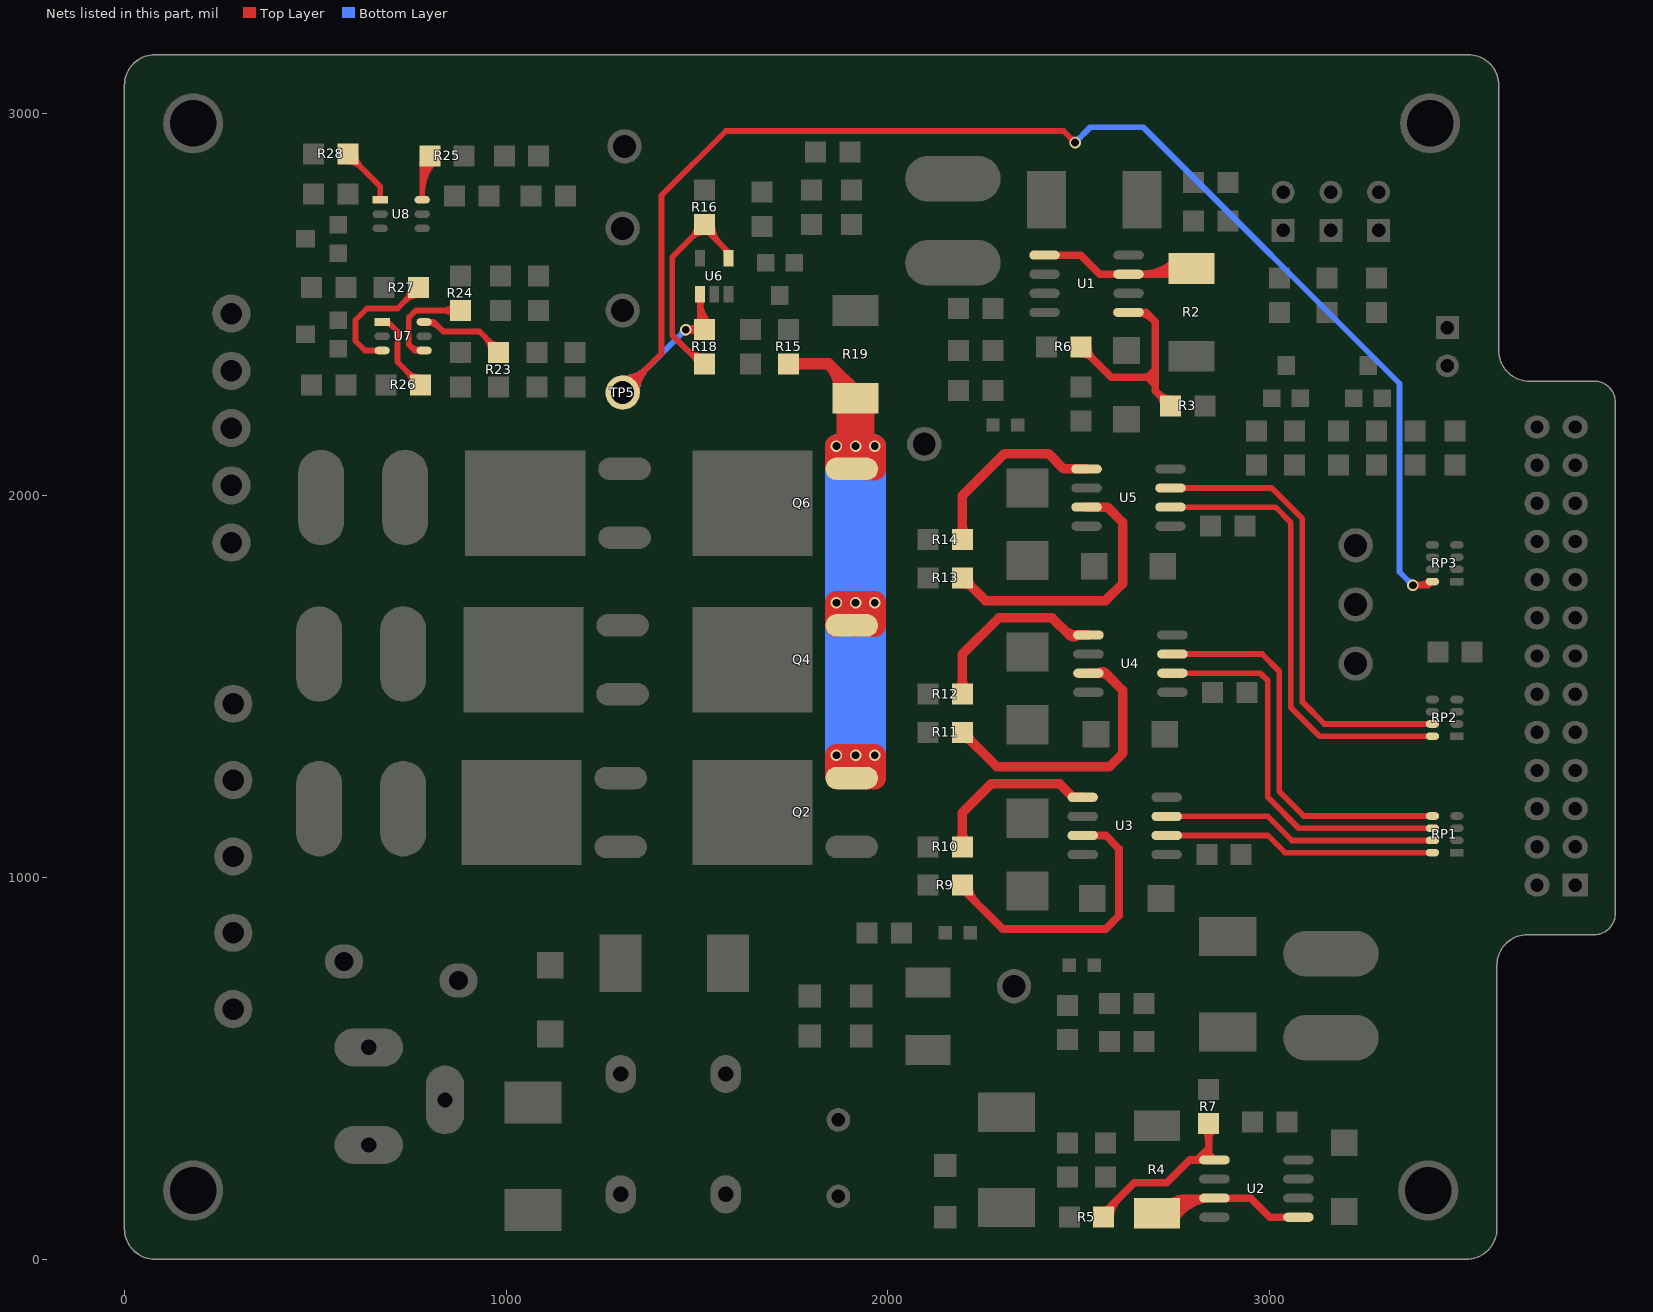
[diagram p0: the nets of this part, all layers, seen from the top]
# Altium PCB MISC103926.PcbDoc (part 4 of 4)
Units mil, origin at the board's own origin, x right, y up, seen from the top; angles counter-clockwise.
Board outline 3905 x 3155 mil, 4 copper layers (Top Layer, GND1, GND2, Bottom Layer); 132 components, 84 nets, 362 pads, 268 vias.

## Via types
v1: diameter 30, hole 20, Top Layer to Bottom Layer, 268 vias

## Nets (pads, with @x,y where several pads share a name; then routed paths per layer and width w, separated by ;. In a path a pad name is that pad's centre, name@x,y a point inside that pad or via, vN(x,y) a via of type N, cw(c..) or ccw(c..) an arc to the next point about the centre after c; other vN are vias at no path point) (continued)
NetQ2_3: Q2.3 Q4.3 Q6.3 R15.2 R19.2 | length 4611.5
  Top Layer w30: R15.2@1740,2345 1845,2345 ; R15.2@1748.84,2336.16 cw(c1770.18,2314.82) 1770.18,2345 cw(c1770.18,2375.18) R15.2@1748.84,2353.84 ; R19.2@1870.51,2260.02 ccw(c1778.82,2278.82) 1845,2345 ; 1884.41,2305.59 cw(c1844.23,2265.41) R19.2@1899.9,2254 ; R19.2@1935,2255 1845,2345
  Top Layer w60: Q2.3@1865,1265 v1(1865,1320) ; Q4.3@1865,1660 v1(1865,1720) ; Q6.3@1865,2075 v1(1865,2130) ; Q2.3@1915,1265 v1(1915,1320) v1(1865,1320) ; Q4.3@1915,1660 v1(1915,1720) v1(1865,1720) ; Q6.3@1915,2075 v1(1915,2130) v1(1865,2130) ; Q2.3@1944.7,1259.98 ccw(c1895.71,1308.98) v1@1965,1308.98 ; Q4.3@1944.7,1659.98 ccw(c1895.71,1708.98) v1@1965,1708.98 ; Q6.3@1944.7,2069.98 ccw(c1895.71,2118.98) v1@1965,2118.98 ; Q2.3@1965,1260 v1(1965,1320) v1(1865,1320) ; Q4.3@1965,1660 v1(1965,1720) v1(1865,1720) ; Q6.3@1965,2070 v1(1965,2130) v1(1865,2130)
  Top Layer w100: v1(1915,2130) R19.2@1915,2245
  Bottom Layer w60: v1@1865,1330 v1(1865,1320) ; 1865,1370 1865,1410 ; 1865,1600 1865,1620 ; 1865,1635 1865,1670 ; v1(1865,1720) v1(1965,1720) v1@1950,1720 ; 1865,1770 1865,1805 ; v1(1915,1320) v1(1915,2130) v1(1865,2130) ; v1(1865,1320) v1(1865,2130) ; v1(1865,1320) v1(1965,1320) v1(1965,2130) v1(1865,2130)
NetR2_2: R2.2 U1.1 U1.7 | length 568.2
  Top Layer w20: U1.1@2410,2630 2505,2630 2555,2580 U1.7@2630,2580 2780,2580 R2.2@2795,2595 ; U1.7@2666.36,2580 ccw(c2666.36,2703.64) R2.2@2753.79,2616.21 ; 2714.64,2580 ccw(c2714.64,2655.36) R2.2@2767.93,2602.07
NetR3_1: R3.1 R6.1 U1.5 | length 810.4
  Top Layer w20: R6.1@2505,2372.5 cw(c2505,2330.25) 2534.87,2360.13 cw(c2564.75,2390) R6.1@2522.5,2390 ; R6.1@2505,2390 2585,2310 2675,2310 ; U1.5@2600,2480 U1.5@2630,2480 2675,2480 2700,2455 2700,2310 ; U1.5@2658,2478 cw(c2658,2432.13) 2690.44,2464.56 ; 2700,2290 2680,2310 ; 2700,2330 2680,2310 ; R3.1@2722.5,2235 ccw(c2680.25,2235) 2710.13,2264.87 ccw(c2740,2294.75) R3.1@2740,2252.5 ; R3.1@2740,2235 2700,2275 2700,2310 ; 2675,2310 2700,2310 ; 2675,2310 2680,2310 ; 2675,2310 2680,2310
NetR4_2: R4.2 U2.1 U2.7 | length 790.7
  Top Layer w20: R4.2@2705,120 2735,120 2775,160 ; R4.2@2716.65,125.5 cw(c2780.71,83.27) 2780.71,160 ; R4.2@2732.99,148.92 ccw(c2744.48,190.51) 2775,160 ; R4.2@2733.35,114.5 cw(c2817.85,58.78) U2.7@2817.85,160 ; R4.2@2750.05,103.49 cw(c2854.99,34.3) U2.7@2855,160 ; R4.2@2755,120 cw(c2803.29,120) 2769.14,154.14 ; U2.1@3075,110 3000,110 2950,160 U2.7@2855,160 ; 2775,160 U2.7@2855,160
NetR5_1: R5.1 R7.1 U2.5 | length 706.3
  Top Layer w20: R5.1@2565,110 2565,120 2645,200 2730,200 2790,260 U2.5@2855,260 2840,275 ; R5.1@2582.5,110 cw(c2648.89,110) 2601.95,156.95 ; 2810,260 2840,290 ; U2.5@2825.8,261.6 ccw(c2804.5,290) 2840,290 ; U2.5@2827,262 ccw(c2827,275) 2840,275 ; R7.1@2827.63,342.63 cw(c2797.75,312.75) 2840,312.75 cw(c2882.25,312.75) R7.1@2852.37,342.63 ; U2.5@2828.99,260.16 cw(c2866.85,263.15) 2840,290 ; R7.1@2840,355 2840,290 ; 2840,275 2840,290
NetR9_1: R9.1 U3.7 | length 814.6
  Top Layer w20: R9.1@2195,980 2195,970 2300,865 2570,865 2605,900 2605,1075 2570,1110 U3.7@2510,1110 ; R9.1@2212.5,980 ccw(c2278.89,980) 2231.95,933.05
NetR10_1: R10.1 U3.5 | length 507.4
  Top Layer w25: R10.1@2184.39,1090.61 ccw(c2158.79,1116.21) 2195,1116.21 ccw(c2231.21,1116.21) R10.1@2205.61,1090.61 ; R10.1@2195,1080 2195,1170 2270,1245 2450,1245 2485,1210 U3.5@2510,1210
NetR11_1: R11.1 U4.7 | length 852.7
  Top Layer w25: R11.1@2195,1365 cw(c2195,1328.79) 2220.61,1354.39 cw(c2246.21,1380) R11.1@2210,1380 ; R11.1@2195,1380 2285,1290 2580,1290 2615,1325 2615,1490 2570,1535 ; U4.7@2525,1535 2570,1535 ; U4.7@2552.66,1535.37 cw(c2561.14,1526.14) 2570,1535 ; U4.7@2553,1535.5 cw(c2553,1495.67) 2581.17,1523.83
NetR12_1: R12.1 U4.5 | length 615.4
  Top Layer w25: R12.1@2184.39,1490.61 ccw(c2158.79,1516.21) 2195,1516.21 ccw(c2231.21,1516.21) R12.1@2205.61,1490.61 ; R12.1@2195,1480 2195,1585 2290,1680 2430,1680 2475,1635 ; 2460.3,1649.7 ccw(c2497,1686.41) U4.5@2497,1634.5 ; U4.5@2497.34,1634.64 cw(c2486.36,1646.36) 2475,1635 ; U4.5@2525,1635 2475,1635
NetR13_1: R13.1 U5.7 | length 791.9
  Top Layer w25: R13.1@2195,1770 cw(c2195,1733.79) 2220.61,1759.39 cw(c2246.21,1785) R13.1@2210,1785 ; R13.1@2195,1785 2255,1725 2570,1725 2615,1770 2615,1930 2575,1970 U5.7@2520,1970
NetR14_1: R14.1 U5.5 | length 559
  Top Layer w25: R14.1@2184.39,1895.61 ccw(c2158.79,1921.21) 2195,1921.21 ccw(c2231.21,1921.21) R14.1@2205.61,1895.61 ; R14.1@2195,1885 2195,2000 2305,2110 2420,2110 2460,2070 U5.5@2520,2070
NetR16_1: R16.1 R18.2 U6.4 | length 851.7
  Top Layer w15: 1468.79,2386.21 ccw(c1520,2437.43) R18.2@1520,2365 ; R18.2@1492.93,2362.07 cw(c1475.86,2345) R18.2@1500,2345 ; R18.2@1494.39,2360.61 ccw(c1520,2386.21) R18.2@1520,2350 ; R16.1@1500,2710 cw(c1451.72,2710) 1485.86,2675.86 cw(c1520,2641.72) 1520,2690 cw(c1520,2665.86) R16.1@1537.07,2682.93 ; R18.2@1520,2345 1510,2345 1435,2420 1435,2625 1515,2705 1582.4,2637.6 U6.4@1582.4,2622.24 ; R16.1@1525,2710 ccw(c1561.21,2710) R16.1@1535.61,2684.39 ; R16.1@1540,2710 ccw(c1612.43,2710) 1561.21,2658.79 ; 1568.77,2651.23 cw(c1548.64,2631.1) U6.4@1577.11,2631.1
NetR18_1: R18.1 RP3.8 TP5.1 U6.1 | length 4789.7
  Top Layer w15: TP5.1@1305,2270 1407,2372 1407,2786.64 1575.36,2955 2460,2955 v1(2490,2925) ; TP5.1@1305,2292.5 ccw(c1305,2346.82) 1343.41,2308.41 ccw(c1381.82,2270) TP5.1@1327.5,2270 ; TP5.1@1305,2307.5 ccw(c1305,2398.03) 1369.02,2334.02 ccw(c1433.03,2270) TP5.1@1342.5,2270 ; v1(1470,2435) R18.1@1520,2435 1507.6,2447.4 U6.1@1507.6,2527.76 ; v1@1473.75,2428.5 cw(c1483.56,2411.51) 1488.64,2430.47 ; v1@1473.75,2441.5 ccw(c1483.56,2458.49) 1488.64,2439.53 ; v1@1475.3,2429.7 cw(c1488.11,2416.89) 1488.11,2435 cw(c1488.11,2453.11) v1@1475.3,2440.3 ; v1@1476.5,2431.25 cw(c1490.86,2422.95) 1486.57,2438.98 ; v1@1476.5,2438.75 ccw(c1490.86,2447.05) 1486.57,2431.02 ; R18.1@1505.86,2420.86 ccw(c1471.72,2386.72) 1471.72,2435 ccw(c1471.72,2483.28) R18.1@1505.86,2449.14 ; 1507.6,2477.01 ccw(c1562.01,2477.01) R18.1@1523.54,2438.54 ; U6.1@1507.6,2513.22 ccw(c1598.22,2513.22) R18.1@1534.14,2449.14 ; 1510.41,2502.75 cw(c1527.6,2507.35) U6.1@1512.18,2516.25 ; v1@2482.5,2925 ccw(c2464.39,2925) 2477.2,2937.8 ccw(c2490,2950.61) v1@2490,2932.5 ; v1(3375,1765) 3416,1765 RP3.8@3426,1775 ; v1@3378.75,1771.5 ccw(c3393.69,1797.37) 3401.42,1768.51 ; v1@3380.3,1759.7 cw(c3393.11,1746.89) 3393.11,1765 cw(c3393.11,1783.11) v1@3380.3,1770.3 ; v1@3388.32,1765 ccw(c3388.32,1805.18) RP3.8@3416.73,1776.77
  Bottom Layer w15: TP5.1@1305,2270 v1(1470,2435) ; TP5.1@1305,2292.5 ccw(c1305,2346.82) 1343.41,2308.41 ccw(c1381.82,2270) TP5.1@1327.5,2270 ; TP5.1@1305,2307.5 ccw(c1305,2398.03) 1369.02,2334.02 ccw(c1433.03,2270) TP5.1@1342.5,2270 ; v1@1462.5,2435 cw(c1444.39,2435) 1457.2,2422.2 cw(c1470,2409.39) v1@1470,2427.5 ; v1(2490,2925) 2530,2965 2668.79,2965 3340,2293.79 3340,1800 v1(3375,1765) ; v1@2490,2932.5 ccw(c2490,2950.61) 2502.8,2937.8 ccw(c2515.61,2925) v1@2497.5,2925 ; v1@3367.5,1765 ccw(c3349.39,1765) 3362.2,1777.8 ccw(c3375,1790.61) v1@3375,1772.5
NetR23_2: R23.2 U7.6 | length 342.2
  Top Layer w15: U7.6@785,2455 810,2455 835,2430 930,2430 R23.2@985,2375 ; U7.6@795,2452.5 cw(c795,2410.25) 824.88,2440.12 ; 942.32,2417.68 cw(c899.64,2375) R23.2@960,2375 ; 954.39,2405.61 ccw(c980,2431.21) R23.2@980,2395
NetR24_2: R24.2 U7.4 | length 369.5
  Top Layer w15: U7.4@774.98,2382.7 cw(c774.7,2424.7) 745,2395 ; U7.4@785,2380.2 759.8,2380.2 745,2395 ; R24.2@865.86,2470.86 ccw(c831.72,2436.72) 831.72,2485 ccw(c831.72,2533.28) R24.2@865.86,2499.14 ; R24.2@880,2485 763.28,2485 745,2466.72 745,2395
NetR25_2: R25.2 U8.6 | length 312.6
  Top Layer w15: U8.6@780,2775 780,2870 R25.2@800,2890 ; 780,2793.43 cw(c896.57,2793.43) R25.2@814.14,2875.86 ; 780,2829.64 cw(c860.36,2829.64) R25.2@803.54,2886.46 ; R25.2@780,2865.86 cw(c824.14,2865.86) R25.2@792.93,2897.07
NetR26_1: R26.1 U7.1 | length 305.3
  Top Layer w15: U7.1@675,2455 690,2455 715,2430 715,2350 R26.1@775,2290 ; U7.1@685,2452.5 cw(c685,2434.39) 697.8,2447.2 ; R26.1@755,2290 ccw(c706.72,2290) 740.86,2324.14 ccw(c775,2358.28) R26.1@775,2310
NetR27_1: R27.1 U7.3 | length 411.3
  Top Layer w15: U7.3@675,2380.2 629.8,2380.2 605,2405 605,2460 635,2490 715,2490 R27.1@770,2545 ; R27.1@750,2545 cw(c701.72,2545) 735.86,2510.86 cw(c770,2476.72) R27.1@770,2525
NetR28_1: R28.1 U8.1 | length 231.1
  Top Layer w15: R28.1@585,2875 cw(c585,2826.72) 619.14,2860.86 cw(c653.28,2895) R28.1@605,2895 ; R28.1@585,2895 670,2810 U8.1@670,2775
NetRP1_5: RP1.5 U4.3 | length 1041.1
  Top Layer w15: U4.3@2745,1585 2980,1585 3025,1540 3025,1225 3089,1161 RP1.5@3426,1161
NetRP1_6: RP1.6 U4.2 | length 1027.8
  Top Layer w15: U4.2@2745,1535 2975,1535 2995,1515 2995,1210 3076,1129 RP1.6@3426,1129
NetRP1_7: RP1.7 U3.3 | length 722.1
  Top Layer w15: U3.3@2730,1160 2995,1160 3058,1097 RP1.7@3426,1097
NetRP1_8: RP1.8 U3.2 | length 714.6
  Top Layer w15: U3.2@2730,1110 2995,1110 3040,1065 RP1.8@3426,1065
NetRP2_7: RP2.7 U5.3 | length 1223.2
  Top Layer w15: U5.3@2740,2020 3005,2020 3085,1940 3085,1460 3143,1402 RP2.7@3426,1402
NetRP2_8: RP2.8 U5.2 | length 1218.6
  Top Layer w15: U5.2@2740,1970 3015,1970 3055,1930 3055,1445 3130,1370 RP2.8@3426,1370
pads on no net: JP1.7 JP1.8 JP1.9 JP1.14 JP1.15 JP1.17 JP1.18 JP1.19 U1.8 U2.8 U8.4

## Polygon pours and split planes (outlines as drawn)
GND on Bottom Layer "Top Layer-No Net" (solid, remove dead copper, pour order 2): 1456.72,-4.27 1456.72,655.73 1206.72,655.73 1206.72,950.73 2506.72,950.73 2506.72,2200.73 926.72,2200.73 806.72,2200.73 356.72,1750.73 346.72,1740.73 1.72,1740.73 1.72,3145.73 -8.28,3155.73 -3.28,3160.73 3911.72,3160.73 3911.72,5.73 3916.72,0.73
GND on Top Layer "Top Layer-No Net 1" (solid, remove dead copper, pour order 6): 1453.51,-8.28 1453.51,641.72 1203.51,641.72 1203.51,946.72 2158.51,946.72 2158.51,2201.72 453.51,2201.72 448.51,2201.72 383.51,2136.72 378.51,2131.72 378.51,1936.72 373.51,1936.72 173.51,1736.72 -46.49,1736.72 -46.49,3186.72 -41.49,3191.72 3958.51,3191.72 3958.51,-13.28
GND on GND2 (split plane): 80,3134.9 3520,3134.9 3520.59,3134.96 3526.72,3134.62 3533.35,3133.49 3539.81,3131.63 3546.03,3129.05 3551.92,3125.8 3557.41,3121.91 3562.42,3117.42 3566.91,3112.41 3570.8,3106.92 3574.05,3101.03 3576.63,3094.81 3578.49,3088.35 3579.62,3081.72 3579.96,3075.59 3579.9,3075 3579.9,2380 3579.91,2379.97 3580.29,2371.28 3581.43,2362.62 3583.32,2354.09 3585.94,2345.77 3589.28,2337.7 3593.31,2329.95 3598.01,2322.59 3603.32,2315.66 3609.22,2309.22 3615.66,2303.32 3622.59,2298.01 3629.95,2293.31 3637.7,2289.28 3645.77,2285.94 3654.09,2283.32 3662.62,2281.43 3671.28,2280.29 3679.97,2279.91 3680,2279.9 3850,2279.9 3850.44,2279.95 3854.57,2279.68 3859.05,2278.78 3863.38,2277.31 3867.49,2275.29 3871.29,2272.75 3874.73,2269.73 3877.75,2266.29 3880.29,2262.49 3882.31,2258.38 3883.78,2254.05 3884.68,2249.57 3884.95,2245.44 3884.9,2245 3884.9,905 3884.95,904.56 3884.68,900.43 3883.78,895.95 3882.31,891.62 3880.29,887.51 3877.75,883.71 3874.73,880.27 3871.29,877.25 3867.49,874.71 3863.38,872.69 3859.05,871.22 3854.57,870.32 3850.44,870.05 3850,870.1 3675,870.1 3674.97,870.09 3666.28,869.71 3657.62,868.57 3649.09,866.68 3640.77,864.06 3632.7,860.72 3624.95,856.69 3617.59,851.99 3610.66,846.68 3604.22,840.78 3598.32,834.34 3593.01,827.41 3588.31,820.05 3584.28,812.3 3580.94,804.23 3578.32,795.91 3576.43,787.38 3575.29,778.72 3574.91,770.03 3574.9,770 3574.9,80 3574.96,79.41 3574.62,73.28 3573.49,66.65 3571.63,60.18 3569.05,53.97 3565.8,48.08 3561.91,42.59 3557.42,37.58 3552.41,33.09 3546.92,29.2 3541.03,25.95 3534.81,23.37 3528.35,21.51 3521.72,20.38 3515.59,20.04 3515,20.1 80,20.1 79.41,20.04 73.28,20.38 66.65,21.51 60.18,23.37 53.97,25.95 48.08,29.2 42.59,33.09 37.58,37.58 33.09,42.59 29.2,48.08 25.95,53.97 23.37,60.19 21.51,66.65 20.38,73.28 20.04,79.41 20.1,80 20.1,3075 20.04,3075.59 20.38,3081.72 21.51,3088.35 23.37,3094.81 25.95,3101.03 29.2,3106.92 33.09,3112.41 37.58,3117.42 42.59,3121.91 48.08,3125.8 53.97,3129.05 60.19,3131.63 66.65,3133.49 73.28,3134.62 79.41,3134.96
GND on GND1 (split plane): 80,3134.9 3520,3134.9 3520.59,3134.96 3526.72,3134.62 3533.35,3133.49 3539.81,3131.63 3546.03,3129.05 3551.92,3125.8 3557.41,3121.91 3562.42,3117.42 3566.91,3112.41 3570.8,3106.92 3574.05,3101.03 3576.63,3094.81 3578.49,3088.35 3579.62,3081.72 3579.96,3075.59 3579.9,3075 3579.9,2380 3579.91,2379.97 3580.29,2371.28 3581.43,2362.62 3583.32,2354.09 3585.94,2345.77 3589.28,2337.7 3593.31,2329.95 3598.01,2322.59 3603.32,2315.66 3609.22,2309.22 3615.66,2303.32 3622.59,2298.01 3629.95,2293.31 3637.7,2289.28 3645.77,2285.94 3654.09,2283.32 3662.62,2281.43 3671.28,2280.29 3679.97,2279.91 3680,2279.9 3850,2279.9 3850.44,2279.95 3854.57,2279.68 3859.05,2278.78 3863.38,2277.31 3867.49,2275.29 3871.29,2272.75 3874.73,2269.73 3877.75,2266.29 3880.29,2262.49 3882.31,2258.38 3883.78,2254.05 3884.68,2249.57 3884.95,2245.44 3884.9,2245 3884.9,905 3884.95,904.56 3884.68,900.43 3883.78,895.95 3882.31,891.62 3880.29,887.51 3877.75,883.71 3874.73,880.27 3871.29,877.25 3867.49,874.71 3863.38,872.69 3859.05,871.22 3854.57,870.32 3850.44,870.05 3850,870.1 3675,870.1 3674.97,870.09 3666.28,869.71 3657.62,868.57 3649.09,866.68 3640.77,864.06 3632.7,860.72 3624.95,856.69 3617.59,851.99 3610.66,846.68 3604.22,840.78 3598.32,834.34 3593.01,827.41 3588.31,820.05 3584.28,812.3 3580.94,804.23 3578.32,795.91 3576.43,787.38 3575.29,778.72 3574.91,770.03 3574.9,770 3574.9,80 3574.96,79.41 3574.62,73.28 3573.49,66.65 3571.63,60.18 3569.05,53.97 3565.8,48.08 3561.91,42.59 3557.42,37.58 3552.41,33.09 3546.92,29.2 3541.03,25.95 3534.81,23.37 3528.35,21.51 3521.72,20.38 3515.59,20.04 3515,20.1 80,20.1 79.41,20.04 73.28,20.38 66.65,21.51 60.18,23.37 53.97,25.95 48.08,29.2 42.59,33.09 37.58,37.58 33.09,42.59 29.2,48.08 25.95,53.97 23.37,60.19 21.51,66.65 20.38,73.28 20.04,79.41 20.1,80 20.1,3075 20.04,3075.59 20.38,3081.72 21.51,3088.35 23.37,3094.81 25.95,3101.03 29.2,3106.92 33.09,3112.41 37.58,3117.42 42.59,3121.91 48.08,3125.8 53.97,3129.05 60.19,3131.63 66.65,3133.49 73.28,3134.62 79.41,3134.96

## Keep-outs
Keep-Out Layer:
  the board outline again, w10

## Other copper
Top Layer:
  rectangle net +24V: 900,1160 1190,1970
Bottom Layer:
  rectangle net MT_PV: 790,1450 1410,1755
  rectangle net MT_PU: 790,1045 1410,1350
  rectangle net MT_PW: 795,1865 1415,2150

## Silkscreen, mask and mechanical layers (free items; w line width, h text height)
Top Overlay:
  circle w16: c343,161 r5
  lines w10: 328.35,141.45 cw(c343.54,161.31) 359.03,141.69
  lines w12: 344,81 344,153 ; 344,188 344,259
  text "W" at 445,2425 h100 r90
  text "V" at 450,2320 h100 r90
  text "U" at 445,2180 h100 r90
  text "GND" at 450,1960 h100 r90
  text "5V" at 450,1805 h100 r90
  text "W" at 445,1400 h100 r90
  text "V" at 445,1225 h100 r90
  text "U" at 440,1035 h100 r90
  text "24V" at 440,825 h100 r90
  text "GND" at 440,505 h100 r90
  text "2013/4/5" at 3525,455 h80 r90
  text "BLDC Driver V1.00" at 3420,310 h80 r90
  text "-" at 327,246 h60 r90
  text "+24V" at 440,90 h80 r90
  text "+" at 300,73 h60
Bottom Overlay:
  lines w10: 3315,1035 3585,1035 ; 3315,1135 3585,1135 ; 3315,1240 3585,1240 ; 3315,1340 3585,1340 ; 3315,1440 3585,1440 ; 3315,1540 3585,1540 ; 3315,1640 3585,1640 ; 3315,1740 3585,1740 ; 3315,1835 3585,1835 ; 3315,1940 3585,1940 ; 3315,2035 3585,2035 ; 3315,2140 3585,2140 ; 3450,930 3450,2235 ; 3315,925 3315,2235 3585,2235 3585,925 3315,925
  text "GND" at 3435,2175 h40
  text "5V" at 3570,2175 h40
  text "A_MW" at 3435,2080 h40
  text "A_MV" at 3570,2075 h40
  text "A_MU" at 3435,1975 h40
  text "A_CU" at 3570,1975 h40
  text "GND" at 3435,1870 h40
  text "NULL" at 3570,1870 h40
  text "NULL" at 3435,1770 h40
  text "NULL" at 3570,1770 h40
  text "GND" at 3435,1675 h40
  text "NULL" at 3570,1675 h40
  text "BLDC Driver V1.00" at 150,1600 h120 r90
  text "NULL" at 3435,1575 h40
  text "H_W" at 3570,1575 h40
  text "H_V" at 3435,1475 h40
  text "H_U" at 3570,1475 h40
  text "GND" at 3435,1375 h40
  text "NULL" at 3570,1375 h40
  text "NULL" at 3430,1270 h40
  text "NULL" at 3565,1270 h40
  text "P_WL" at 3430,1170 h40
  text "P_WH" at 3565,1170 h40
  text "P_VL" at 3430,1075 h40
  text "P_VH" at 3565,1075 h40
  text "P_UL" at 3430,975 h40
  text "P_UH" at 3565,975 h40
  text "2013/4/5" at 810,60 h120